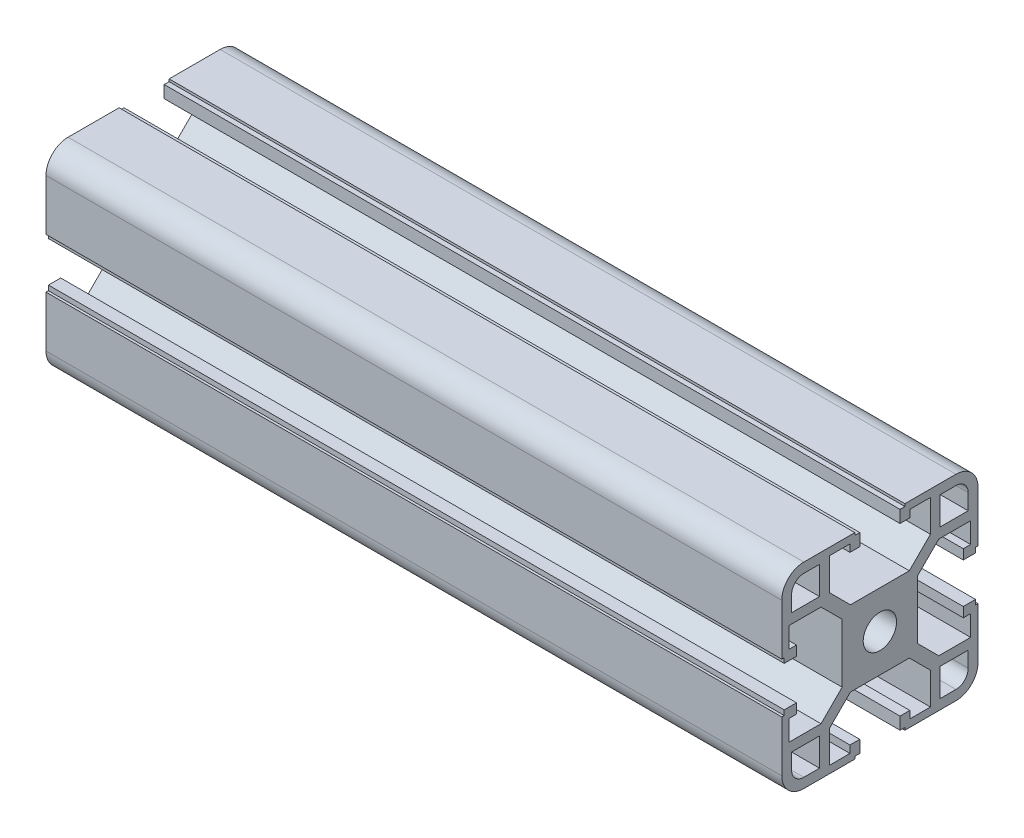
from build123d import *

# Parameters (mm, degrees)
SKETCH1_R                                 = 3.4
ALUMINIUM_PROFILE_40_X_40B_X_R4_5_1_DEPTH = 150


with BuildPart() as part:
    # Sketch1 → Aluminium profile 40 X 40B X R4.5(1) (new body)
    with BuildSketch(Plane.YZ.offset(-984.974958264)):
        with BuildLine():
            Line((-5.1, 20), (-5.1, 19.5))
            Line((-5.1, 19.5), (-4.1, 19.5))
            Line((-4.1, 19.5), (-4.1, 17))
            Line((-4.1, 17), (-6.1, 17))
            Line((-6.1, 17), (-6.1, 18.5))
            Line((-6.1, 18.5), (-10.3, 18.5))
            Line((-10.3, 18.5), (-10.3, 12))
            Line((-10.3, 12), (-6, 7.7))
            Line((-6, 7.7), (6, 7.7))
            Line((6, 7.7), (10.3, 12))
            Line((10.3, 12), (10.3, 18.5))
            Line((10.3, 18.5), (6.1, 18.5))
            Line((6.1, 18.5), (6.1, 17))
            Line((6.1, 17), (4.1, 17))
            Line((4.1, 17), (4.1, 19.5))
            Line((4.1, 19.5), (5.1, 19.5))
            Line((5.1, 19.5), (5.1, 20))
            Line((5.1, 20), (15.5, 20))
            ThreePointArc((15.5, 20), (18.681980515, 18.681980515), (20, 15.5))
            Line((20, 15.5), (20, 5.1))
            Line((20, 5.1), (19.5, 5.1))
            Line((19.5, 5.1), (19.5, 4.1))
            Line((19.5, 4.1), (17, 4.1))
            Line((17, 4.1), (17, 6.1))
            Line((17, 6.1), (18.5, 6.1))
            Line((18.5, 6.1), (18.5, 10.3))
            Line((18.5, 10.3), (12, 10.3))
            Line((12, 10.3), (7.7, 6))
            Line((7.7, 6), (7.7, -6))
            Line((7.7, -6), (12, -10.3))
            Line((12, -10.3), (18.5, -10.3))
            Line((18.5, -10.3), (18.5, -6.1))
            Line((18.5, -6.1), (17, -6.1))
            Line((17, -6.1), (17, -4.1))
            Line((17, -4.1), (19.5, -4.1))
            Line((19.5, -4.1), (19.5, -5.1))
            Line((19.5, -5.1), (20, -5.1))
            Line((20, -5.1), (20, -15.5))
            ThreePointArc((20, -15.5), (18.681980515, -18.681980515), (15.5, -20))
            Line((15.5, -20), (5.1, -20))
            Line((5.1, -20), (5.1, -19.5))
            Line((5.1, -19.5), (4.1, -19.5))
            Line((4.1, -19.5), (4.1, -17))
            Line((4.1, -17), (6.1, -17))
            Line((6.1, -17), (6.1, -18.5))
            Line((6.1, -18.5), (10.3, -18.5))
            Line((10.3, -18.5), (10.3, -12))
            Line((10.3, -12), (6, -7.7))
            Line((6, -7.7), (-6, -7.7))
            Line((-6, -7.7), (-10.3, -12))
            Line((-10.3, -12), (-10.3, -18.5))
            Line((-10.3, -18.5), (-6.1, -18.5))
            Line((-6.1, -18.5), (-6.1, -17))
            Line((-6.1, -17), (-4.1, -17))
            Line((-4.1, -17), (-4.1, -19.5))
            Line((-4.1, -19.5), (-5.1, -19.5))
            Line((-5.1, -19.5), (-5.1, -20))
            Line((-5.1, -20), (-15.5, -20))
            ThreePointArc((-15.5, -20), (-18.681980515, -18.681980515), (-20, -15.5))
            Line((-20, -15.5), (-20, -5.1))
            Line((-20, -5.1), (-19.5, -5.1))
            Line((-19.5, -5.1), (-19.5, -4.1))
            Line((-19.5, -4.1), (-17, -4.1))
            Line((-17, -4.1), (-17, -6.1))
            Line((-17, -6.1), (-18.5, -6.1))
            Line((-18.5, -6.1), (-18.5, -10.3))
            Line((-18.5, -10.3), (-12, -10.3))
            Line((-12, -10.3), (-7.7, -6))
            Line((-7.7, -6), (-7.7, 6))
            Line((-7.7, 6), (-12, 10.3))
            Line((-12, 10.3), (-18.5, 10.3))
            Line((-18.5, 10.3), (-18.5, 6.1))
            Line((-18.5, 6.1), (-17, 6.1))
            Line((-17, 6.1), (-17, 4.1))
            Line((-17, 4.1), (-19.5, 4.1))
            Line((-19.5, 4.1), (-19.5, 5.1))
            Line((-19.5, 5.1), (-20, 5.1))
            Line((-20, 5.1), (-20, 15.5))
            ThreePointArc((-20, 15.5), (-18.681980515, 18.681980515), (-15.5, 20))
            Line((-15.5, 20), (-5.1, 20))
        make_face()
        Circle(SKETCH1_R, mode=Mode.SUBTRACT)
        with BuildLine():
            Line((12.3, 18), (15.5, 18))
            ThreePointArc((15.5, 18), (17.267766953, 17.267766953), (18, 15.5))
            Line((18, 15.5), (18, 12.3))
            Line((18, 12.3), (12.3, 12.3))
            Line((12.3, 12.3), (12.3, 18))
        make_face(mode=Mode.SUBTRACT)
        with BuildLine():
            Line((-15.5, 18), (-12.3, 18))
            Line((-12.3, 18), (-12.3, 12.3))
            Line((-12.3, 12.3), (-18, 12.3))
            Line((-18, 12.3), (-18, 15.5))
            ThreePointArc((-18, 15.5), (-17.267766953, 17.267766953), (-15.5, 18))
        make_face(mode=Mode.SUBTRACT)
        with BuildLine():
            Line((-18, -12.3), (-12.3, -12.3))
            Line((-12.3, -12.3), (-12.3, -18))
            Line((-12.3, -18), (-15.5, -18))
            ThreePointArc((-15.5, -18), (-17.267766953, -17.267766953), (-18, -15.5))
            Line((-18, -15.5), (-18, -12.3))
        make_face(mode=Mode.SUBTRACT)
        with BuildLine():
            Line((12.3, -12.3), (18, -12.3))
            Line((18, -12.3), (18, -15.5))
            ThreePointArc((18, -15.5), (17.267766953, -17.267766953), (15.5, -18))
            Line((15.5, -18), (12.3, -18))
            Line((12.3, -18), (12.3, -12.3))
        make_face(mode=Mode.SUBTRACT)
    extrude(amount=ALUMINIUM_PROFILE_40_X_40B_X_R4_5_1_DEPTH)


solid = part.part
